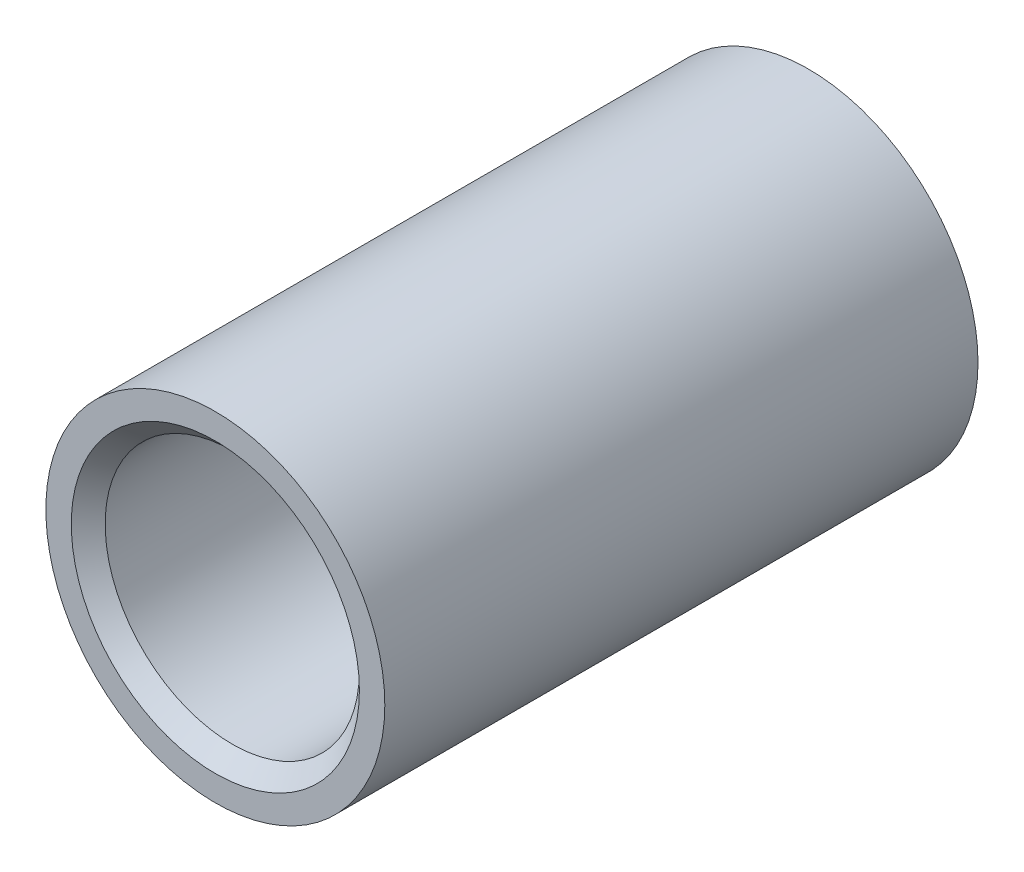
SolidWorks part; units mm, degrees
ref_plane "Front Plane" through (0, 0, 0) normal (0, 0, 1) x (1, 0, 0)
ref_plane "Top Plane" through (0, 0, 0) normal (0, 1, 0) x (1, 0, 0)
ref_plane "Right Plane" through (0, 0, 0) normal (1, 0, 0) x (0, 0, -1)
other "Configuration Table"
sketch "Sketch1" plane through (0, 0, 0) normal (0, 0, 1) x (1, 0, 0)
  circle A0 centre (0, 0) radius 7.5
  circle A1 centre (0, 0) radius 10
  dimension "D1" = 15
  dimension "D2" = 20
extrude "Boss-Extrude1" add sketch "Sketch1" along normal blind 35
chamfer "Chamfer1" distance 1 angle 45 2 edges at (7.5, 0, 0) (7.5, 0, 35)
